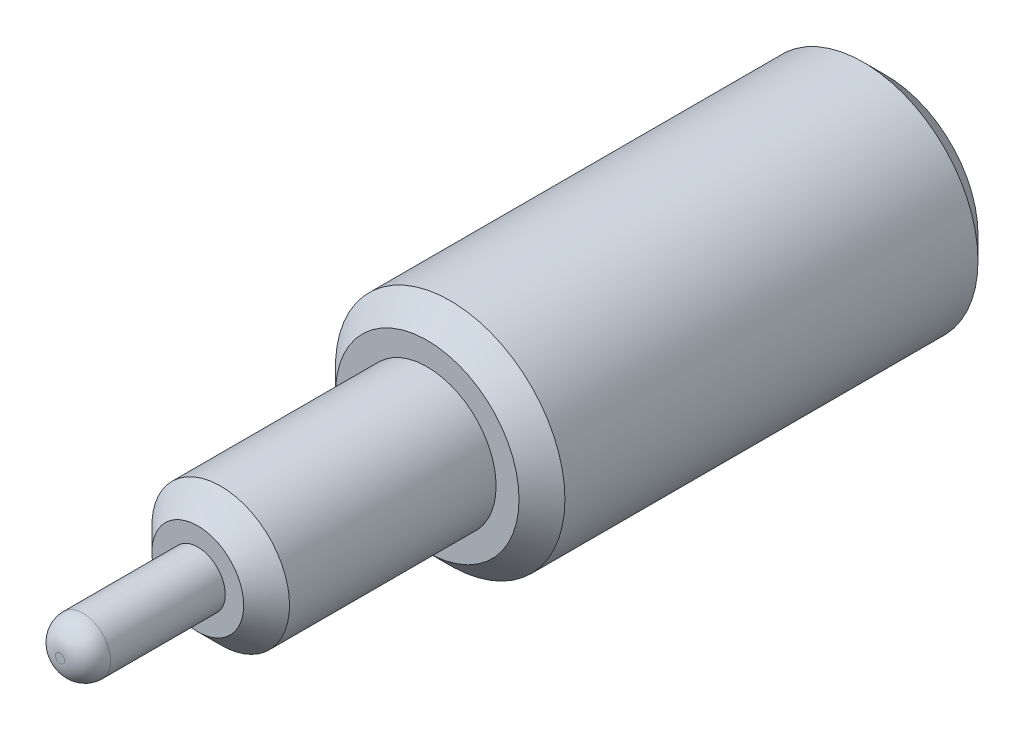
from build123d import *

# Parameters (mm, degrees)
SKETCH1_R           = 2.5
BOSS_EXTRUDE1_DEPTH = 10
SKETCH2_R           = 1.5
BOSS_EXTRUDE2_DEPTH = 5
SKETCH3_R           = 0.6
BOSS_EXTRUDE3_DEPTH = 3
FILLET1_R           = 0.5
SKETCH4_R           = 0.892356389
CUT_EXTRUDE1_DEPTH  = 13
CHAMFER1_SIZE       = 0.5


with BuildPart() as part:
    # Sketch1 → Boss-Extrude1 (new body)
    with BuildSketch(Plane.XY):
        Circle(SKETCH1_R)
    extrude(amount=BOSS_EXTRUDE1_DEPTH)

    # Sketch2 → Boss-Extrude2 (add)
    with BuildSketch(Plane.XY.offset(10)):
        Circle(SKETCH2_R)
    extrude(amount=BOSS_EXTRUDE2_DEPTH)

    # Sketch3 → Boss-Extrude3 (add)
    with BuildSketch(Plane.XY.offset(15)):
        Circle(SKETCH3_R)
    extrude(amount=BOSS_EXTRUDE3_DEPTH)

    # Fillet1
    fillet1_edges = [part.edges().sort_by_distance(p)[0] for p in [
        (-0.6, 0, 18),
    ]]
    fillet(fillet1_edges, radius=FILLET1_R)

    # Sketch4 → Cut-Extrude1 (cut)
    with BuildSketch(Plane(origin=(0, 0, 0), x_dir=(-1, 0, 0), z_dir=(0, 0, -1))):
        Circle(SKETCH4_R)
    extrude(amount=-CUT_EXTRUDE1_DEPTH, mode=Mode.SUBTRACT)

    # Chamfer1
    chamfer1_edges = [part.edges().sort_by_distance(p)[0] for p in [
        (-2.5, 0, 0),
        (-2.5, 0, 10),
        (-1.5, 0, 15),
    ]]
    chamfer(chamfer1_edges, length=CHAMFER1_SIZE)


solid = part.part
